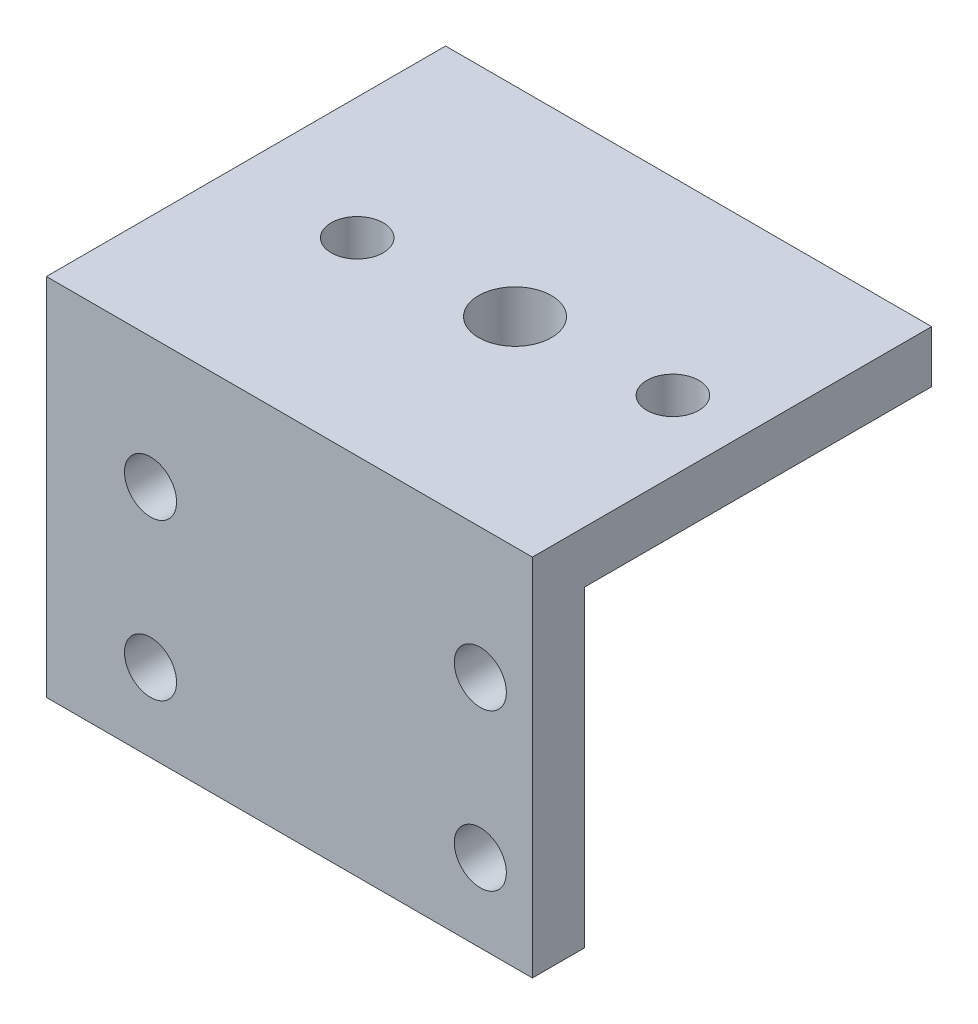
from build123d import *

# Parameters (mm, degrees)
SKETCH1_W           = 25
SKETCH1_H           = 18
SKETCH1_R           = 1.5
BOSS_EXTRUDE1_DEPTH = 3
SKETCH2_W           = 25
SKETCH2_H           = 23
SKETCH2_R           = 2.1
SKETCH2_R_2         = 1.5
BOSS_EXTRUDE2_DEPTH = 3
SKETCH3_W           = 23
SKETCH3_H           = 21
BOSS_EXTRUDE3_DEPTH = 3


with BuildPart() as part:
    # Sketch1 → Boss-Extrude1 (new body)
    with BuildSketch(Plane.XY):
        Rectangle(SKETCH1_W, SKETCH1_H)
        with Locations((-9.5, 4.5)):
            Circle(SKETCH1_R, mode=Mode.SUBTRACT)
        with Locations((9.5, 4.5)):
            Circle(SKETCH1_R, mode=Mode.SUBTRACT)
        with Locations((9.5, -4.5)):
            Circle(SKETCH1_R, mode=Mode.SUBTRACT)
        with Locations((-9.5, -4.5)):
            Circle(SKETCH1_R, mode=Mode.SUBTRACT)
    extrude(amount=BOSS_EXTRUDE1_DEPTH)

    # Sketch2 → Boss-Extrude2 (add)
    with BuildSketch(Plane(origin=(0, 9, 0), x_dir=(1, 0, 0), z_dir=(0, 1, 0))):
        with Locations((0, 8.5)):
            Rectangle(SKETCH2_W, SKETCH2_H)
        with Locations(Location((0, 8.5, 0), (0, 0, 270))):
            Circle(SKETCH2_R, mode=Mode.SUBTRACT)
        with Locations(Location((-8.477677472, 7.884382628, 0), (0, 0, 270))):
            Circle(SKETCH2_R_2, mode=Mode.SUBTRACT)
        with Locations(Location((8.477677464, 9.115617375, 0), (0, 0, 270))):
            Circle(SKETCH2_R_2, mode=Mode.SUBTRACT)
    extrude(amount=BOSS_EXTRUDE2_DEPTH)

    # Sketch3 → Boss-Extrude3 (add)
    with BuildSketch(Plane.ZY.offset(12.5)):
        with Locations((-8.5, 1.5)):
            Rectangle(SKETCH3_W, SKETCH3_H)
    extrude(amount=BOSS_EXTRUDE3_DEPTH)


solid = part.part
